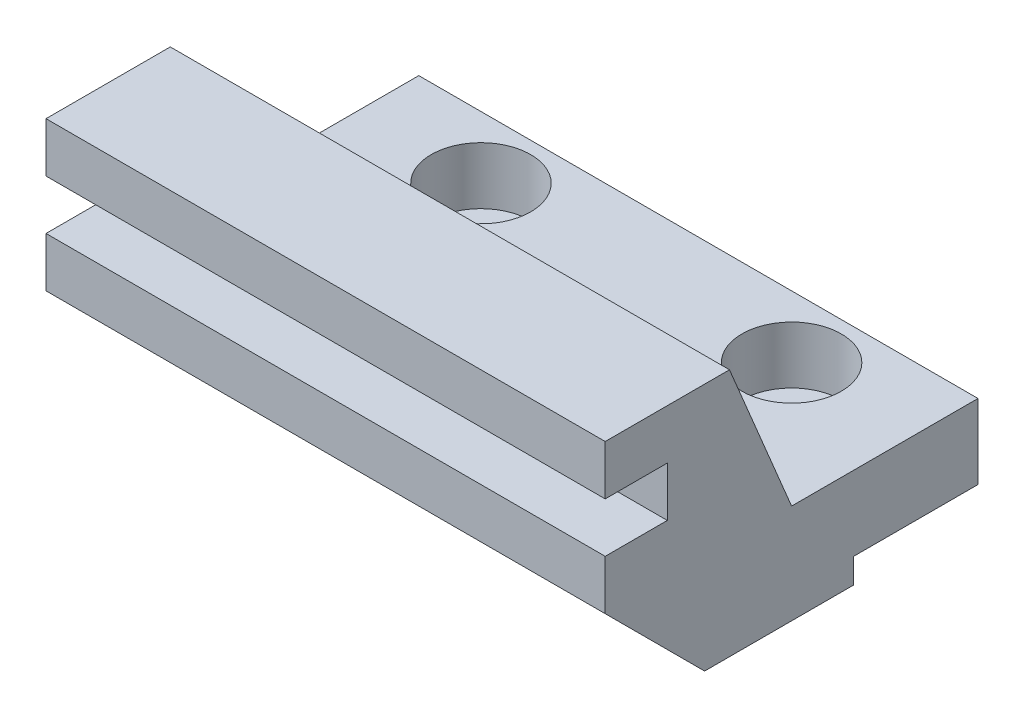
from build123d import *

# Parameters (mm, degrees)
SKETCH1_W                                        = 45
SKETCH1_H                                        = 20
BOSS_EXTRUDE1_DEPTH                              = 30
CUT_EXTRUDE1_DEPTH                               = 56
CUT_EXTRUDE1_DEPTH_BACK                          = 56
SKETCH2_W                                        = 5
SKETCH2_H                                        = 4
CHAMFER1_SIZE                                    = 8
HOLE_FOR_SOCKET_HEAD_CAP_SCREW_TYPE1_D           = 4.5
HOLE_FOR_SOCKET_HEAD_CAP_SCREW_TYPE1_CBORE_D     = 8
HOLE_FOR_SOCKET_HEAD_CAP_SCREW_TYPE1_CBORE_DEPTH = 4.6
CUT_EXTRUDE2_DEPTH                               = 56
CUT_EXTRUDE2_DEPTH_BACK                          = 56
SKETCH7_W                                        = 10
SKETCH7_H                                        = 2


with BuildPart() as part:
    # Sketch1 → Boss-Extrude1 (new body)
    with BuildSketch(Plane.XY):
        Rectangle(SKETCH1_W, SKETCH1_H)
    extrude(amount=BOSS_EXTRUDE1_DEPTH)

    # Sketch2 → Cut-Extrude1 (cut, two sides: drawn at the far end of the back side and taken through both)
    with BuildSketch(Plane.ZY.offset(22.5).offset(-CUT_EXTRUDE1_DEPTH_BACK)):
        Polygon((0, -2), (15, -2), (20, 10), (0, 10), align=None)
        with Locations((27.5, 4)):
            Rectangle(SKETCH2_W, SKETCH2_H)
    extrude(amount=CUT_EXTRUDE1_DEPTH + CUT_EXTRUDE1_DEPTH_BACK, mode=Mode.SUBTRACT)

    # Chamfer1
    chamfer1_edges = [part.edges().sort_by_distance(p)[0] for p in [
        (0, -10, 30),
    ]]
    chamfer(chamfer1_edges, length=CHAMFER1_SIZE)

    # Hole for socket head cap screw, type1 (through all)
    with Locations(Plane(origin=(0, -2, 0), x_dir=(1, 0, 0), z_dir=(0, 1, 0))):
        with Locations((-12.5, -5), (12.5, -5)):
            CounterBoreHole(HOLE_FOR_SOCKET_HEAD_CAP_SCREW_TYPE1_D / 2, HOLE_FOR_SOCKET_HEAD_CAP_SCREW_TYPE1_CBORE_D / 2, HOLE_FOR_SOCKET_HEAD_CAP_SCREW_TYPE1_CBORE_DEPTH)

    # Sketch7 → Cut-Extrude2 (cut, two sides: drawn at the far end of the back side and taken through both)
    with BuildSketch(Plane.ZY.offset(22.5).offset(-CUT_EXTRUDE2_DEPTH_BACK)):
        with Locations((5, -9)):
            Rectangle(SKETCH7_W, SKETCH7_H)
    extrude(amount=CUT_EXTRUDE2_DEPTH + CUT_EXTRUDE2_DEPTH_BACK, mode=Mode.SUBTRACT)


solid = part.part
